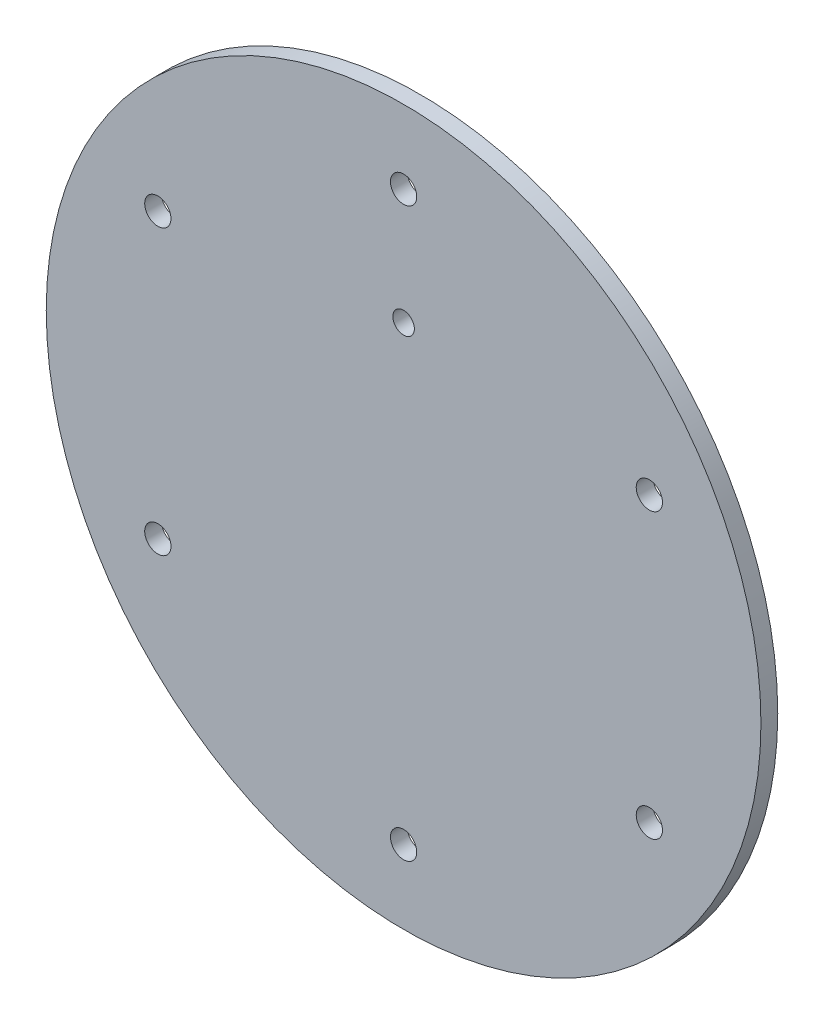
SolidWorks part; units mm, degrees
material "Q235B"
ref_plane "Front Plane" through (0, 0, 0) normal (0, 0, 1) x (1, 0, 0)
ref_plane "Top Plane" through (0, 0, 0) normal (0, 1, 0) x (1, 0, 0)
ref_plane "Right Plane" through (0, 0, 0) normal (1, 0, 0) x (0, 0, -1)
sketch "Sketch1" plane through (0, 0, 0) normal (0, 0, 1) x (1, 0, 0)
  circle A0 centre (0, 0) radius 170
  dimension "D1" = 340
extrude "Boss-Extrude1" add sketch "Sketch1" along normal blind 8
sketch "Sketch3" plane through (0, 0, 0) normal (0, 0, -1) x (-1, 0, 0)
  circle A0 centre (116.9134, 67.5) radius 6.25
  circle A1 centre (0, 135) radius 6.25
  circle A5 centre (116.9134, -67.5) radius 6.25
  circle A6 centre (0, -135) radius 6.25
  circle A7 centre (-116.9134, -67.5) radius 6.25
  circle A8 centre (-116.9134, 67.5) radius 6.25
  point P14 (0, 0)
  point P22 (0, 0)
  dimension "D1" = 12.5
  dimension "D2" = 6
  dimension "D3" = 135
extrude "Cut-Extrude1" cut sketch "Sketch3" against normal blind 10
sketch "Sketch4" plane through (0, 0, 0) normal (0, 0, -1) x (-1, 0, 0)
  circle A0 centre (0, 80) radius 5.125
  dimension "D1" = 10.25
  dimension "D2" = 80
extrude "Cut-Extrude2" cut sketch "Sketch4" against normal blind 10
